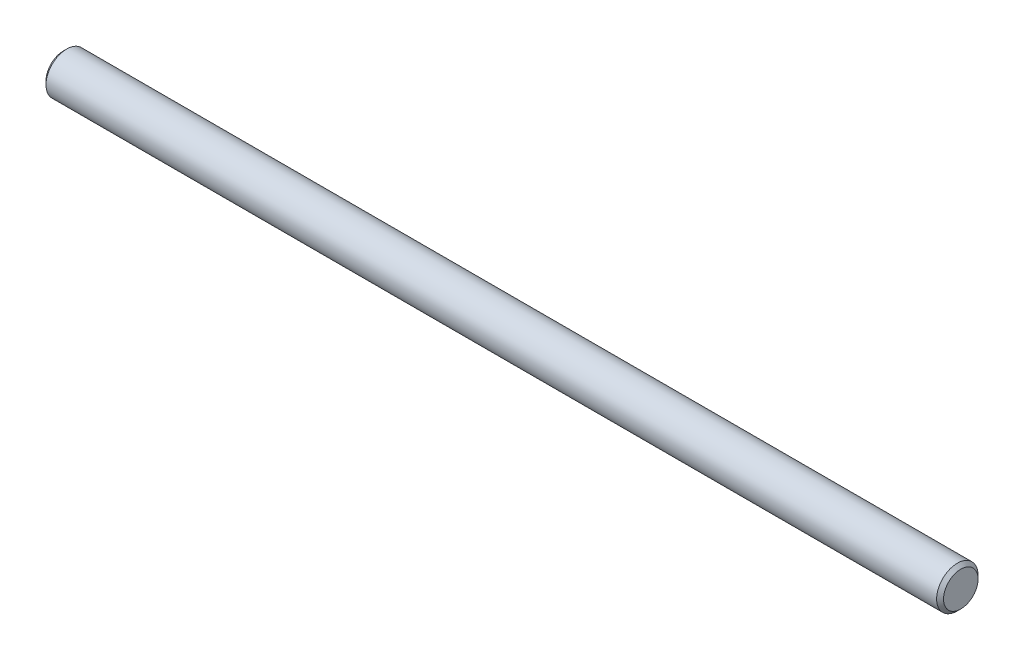
from build123d import *

# Parameters (mm, degrees)
SKETCH1_W     = 130
SKETCH1_H     = 3
CHAMFER1_SIZE = 0.5


with BuildPart() as part:
    # Sketch1 → Revolve1 (revolve)
    with BuildSketch(Plane.XY, mode=Mode.PRIVATE) as revolve1_sk:
        with Locations((65, 1.5)):
            Rectangle(SKETCH1_W, SKETCH1_H)
    revolve(revolve1_sk.sketch.rotate(Axis((0, 0, 0), (1, 0, 0)), 90), axis=Axis((0, 0, 0), (1, 0, 0)))

    # Chamfer1
    chamfer1_edges = [part.edges().sort_by_distance(p)[0] for p in [
        (130, 0, -3),
        (0, 0, -3),
    ]]
    chamfer(chamfer1_edges, length=CHAMFER1_SIZE)


solid = part.part
